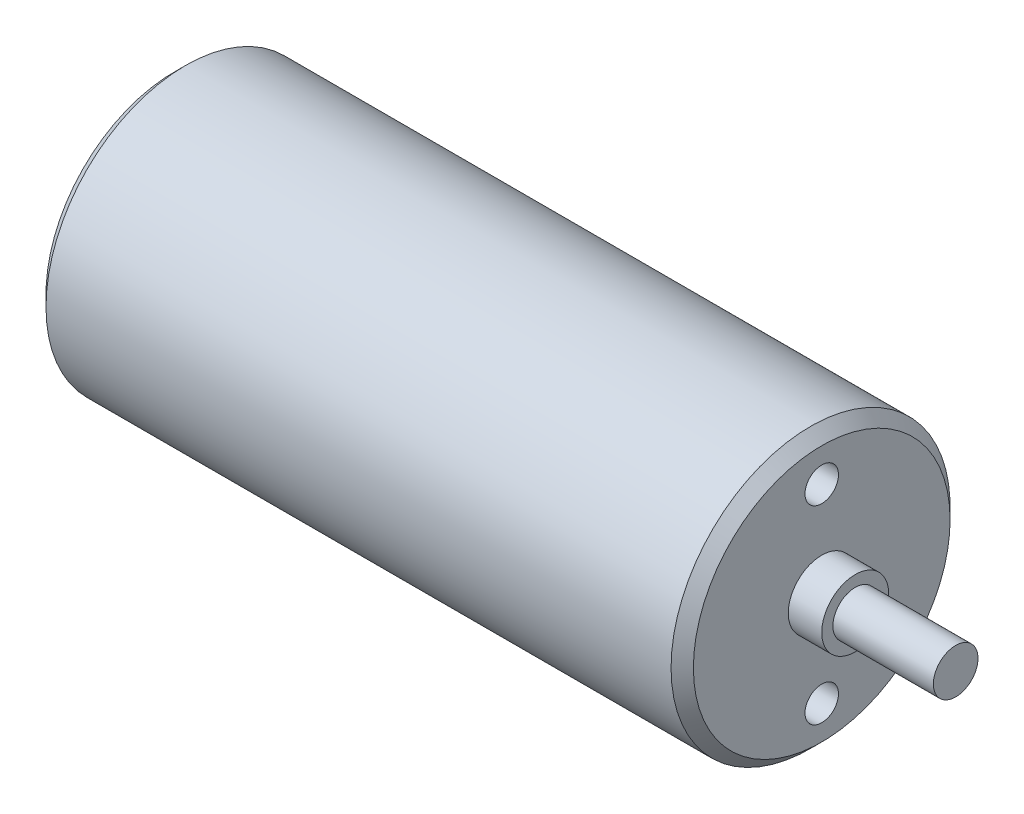
from build123d import *

# Parameters (mm, degrees)
SKETCH1_R           = 12.5
BOSS_EXTRUDE1_DEPTH = 58
SKETCH2_R           = 3
BOSS_EXTRUDE2_DEPTH = 3
SKETCH3_R           = 2
BOSS_EXTRUDE3_DEPTH = 9
SKETCH4_R           = 1.5
CUT_EXTRUDE1_DEPTH  = 6
CHAMFER1_SIZE       = 1
CHAMFER2_SIZE       = 1


with BuildPart() as part:
    # Sketch1 → Boss-Extrude1 (new body)
    with BuildSketch(Plane(origin=(0, 0, 0), x_dir=(0, 0, -1), z_dir=(1, 0, 0))):
        with Locations(Location((0, 0, 0), (0, 0, 180))):
            Circle(SKETCH1_R)
    extrude(amount=BOSS_EXTRUDE1_DEPTH)

    # Sketch2 → Boss-Extrude2 (add)
    with BuildSketch(Plane(origin=(58, 0, 0), x_dir=(0, 0, -1), z_dir=(1, 0, 0))):
        Circle(SKETCH2_R)
    extrude(amount=BOSS_EXTRUDE2_DEPTH)

    # Sketch3 → Boss-Extrude3 (add)
    with BuildSketch(Plane(origin=(61, 0, 0), x_dir=(0, 0, -1), z_dir=(1, 0, 0))):
        Circle(SKETCH3_R)
    extrude(amount=BOSS_EXTRUDE3_DEPTH)

    # Sketch4 → Cut-Extrude1 (cut)
    with BuildSketch(Plane(origin=(58, 0, 0), x_dir=(0, 0, -1), z_dir=(1, 0, 0))):
        with Locations((0, 8.5)):
            Circle(SKETCH4_R)
        with Locations(Location((0, -8.5, 0), (0, 0, 180))):
            Circle(SKETCH4_R)
    extrude(amount=-CUT_EXTRUDE1_DEPTH, mode=Mode.SUBTRACT)

    # Chamfer1
    chamfer1_edges = [part.edges().sort_by_distance(p)[0] for p in [
        (58, 0, -12.5),
    ]]
    chamfer(chamfer1_edges, length=CHAMFER1_SIZE)

    # Chamfer2
    chamfer2_edges = [part.edges().sort_by_distance(p)[0] for p in [
        (0, 0, -12.5),
    ]]
    chamfer(chamfer2_edges, length=CHAMFER2_SIZE)


solid = part.part
